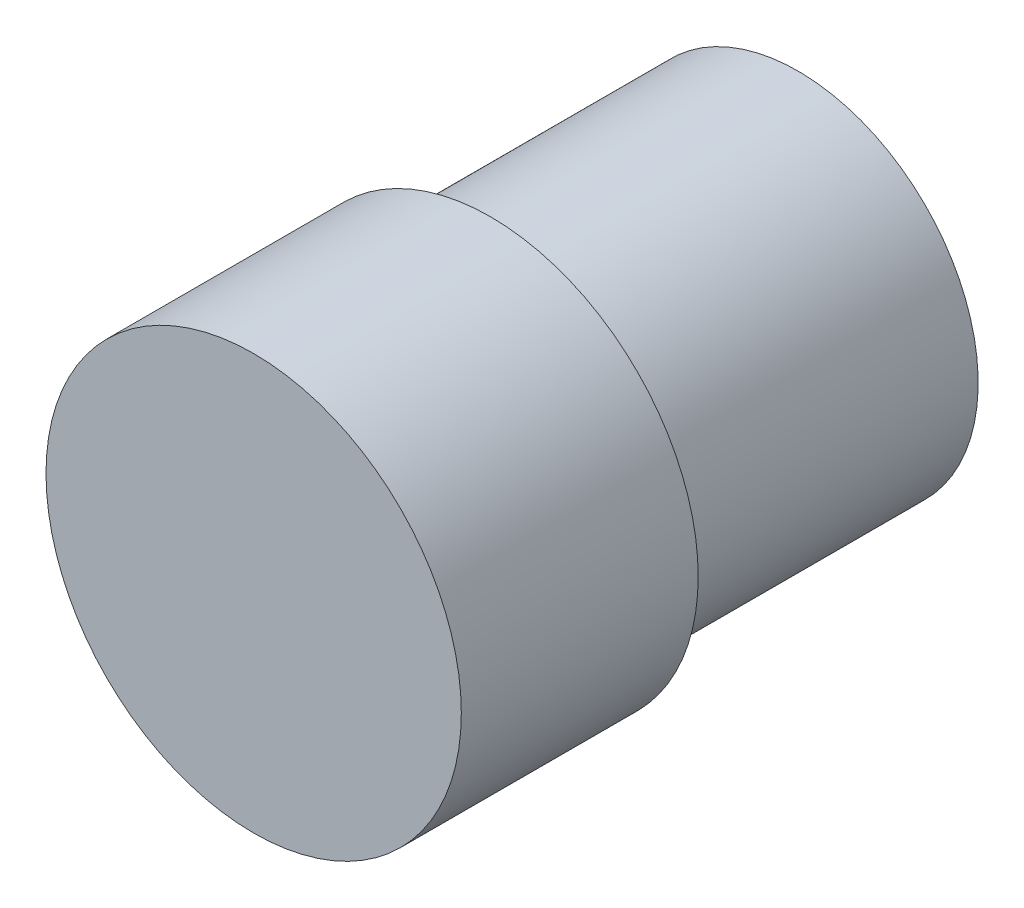
from build123d import *

# Parameters (mm, degrees)
SKETCH1_R           = 6.75
BOSS_EXTRUDE1_DEPTH = 4.5
BOSS_EXTRUDE2_START = 3.2
SKETCH2_R           = 6.75
BOSS_EXTRUDE2_DEPTH = 3.2
SKETCH3_R           = 5.85
BOSS_EXTRUDE3_DEPTH = 10


with BuildPart() as part:
    # Sketch1 → Boss-Extrude1 (new body)
    with BuildSketch(Plane.XY):
        with Locations((50.531925728, -8.105666666)):
            Circle(SKETCH1_R)
    extrude(amount=BOSS_EXTRUDE1_DEPTH)

    # Sketch2 → Boss-Extrude2 (add)
    with BuildSketch(Plane(origin=(0, 0, 0), x_dir=(-1, 0, 0), z_dir=(0, 0, -1)).offset(BOSS_EXTRUDE2_START)):
        with Locations((-50.531925728, -8.105666666)):
            Circle(SKETCH2_R)
    extrude(amount=-BOSS_EXTRUDE2_DEPTH)

    # Sketch3 → Boss-Extrude3 (add)
    with BuildSketch(Plane(origin=(0, 0, -3.2), x_dir=(-1, 0, 0), z_dir=(0, 0, -1))):
        with Locations((-50.531925728, -8.105666666)):
            Circle(SKETCH3_R)
    extrude(amount=BOSS_EXTRUDE3_DEPTH)


solid = part.part
